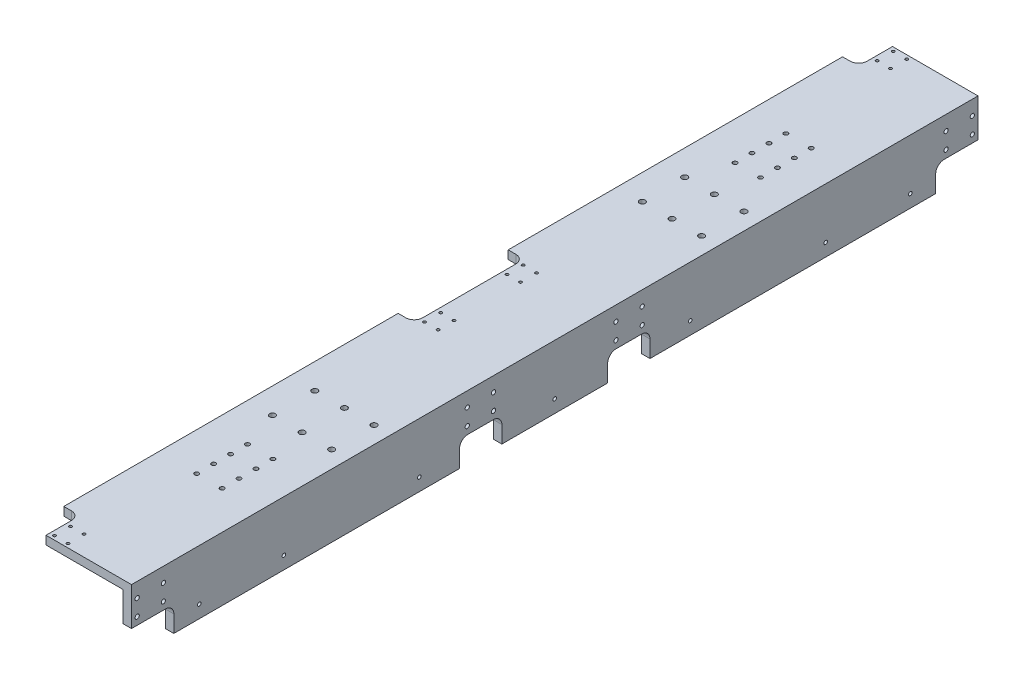
from build123d import *

# Parameters (mm, degrees)
EXTRUDE_1_DEPTH     = 500
HOLE_WIZARD_M8_1_D  = 6.8
MOVE_FACE_1_BY      = 20
MOVE_FACE_2_BY      = 15
CHAMFER_1_SIZE      = 10
SKETCH_16_W         = 19
SKETCH_16_H         = 40
SKETCH_16_H_2       = 130
CUT_EXTRUDE_1_DEPTH = 516.388203202
SKETCH_17_W         = 50
SKETCH_17_H         = 30
CUT_EXTRUDE_2_DEPTH = 520.639297975
HOLE_WIZARD_M6_1_D  = 5
HOLE_WIZARD_M4_1_D  = 3.3
HOLE_WIZARD_M5_3_D  = 4.2
HOLE_WIZARD_M6_2_D  = 5
FILLET_1_R          = 10


with BuildPart() as part:
    # 草图1 → 凸台-拉伸1 (new, symmetric)
    with BuildSketch(Plane.XY):
        Polygon((0, 0), (100, 0), (100, -90), (90, -90), (90, -10), (0, -10), align=None)
    extrude(amount=EXTRUDE_1_DEPTH, both=True)

    # M8 螺纹孔1 (through all)
    with Locations(Plane(origin=(0, 0, 0), x_dir=(1, 0, 0), z_dir=(0, 1, 0))):
        with Locations((10, -193.5), (10, -243.5), (80, -193.5), (80, -243.5), (45, -243.5), (45, -193.5), (45, 193.5), (45, 243.5), (80, 243.5), (80, 193.5), (10, 243.5), (10, 193.5)):
            Hole(HOLE_WIZARD_M8_1_D / 2)

    # Move Face 1: a face moved outward by 20.0
    extrude(part.faces().sort_by_distance((0, -5, 0))[0], amount=MOVE_FACE_1_BY, dir=(-1, 0, 0))

    # Move Face 2: a face moved inward by 15.0
    extrude(part.faces().sort_by_distance((95, -90, 0))[0], amount=MOVE_FACE_2_BY, dir=(0, 1, 0), mode=Mode.SUBTRACT)

    # 倒角1
    chamfer_1_edges = [part.edges().sort_by_distance(p)[0] for p in [
        (95, -75, 500),
        (-20, -5, 500),
        (95, -75, -500),
        (-20, -5, -500),
    ]]
    chamfer(chamfer_1_edges, length=CHAMFER_1_SIZE)

    # 草图16 → 切除-拉伸1 (cut, through all)
    with BuildSketch(Plane(origin=(0, 0, 0), x_dir=(1, 0, 0), z_dir=(0, 1, 0))):
        with Locations((-10.5, -480)):
            Rectangle(SKETCH_16_W, SKETCH_16_H)
        with Locations((-10.5, 480)):
            Rectangle(SKETCH_16_W, SKETCH_16_H)
        with Locations((-10.5, 0)):
            Rectangle(SKETCH_16_W, SKETCH_16_H_2)
    extrude(amount=-CUT_EXTRUDE_1_DEPTH, mode=Mode.SUBTRACT)

    # 草图17 → 切除-拉伸2 (cut, through all)
    with BuildSketch(Plane(origin=(100, 0, 0), x_dir=(0, 0, -1), z_dir=(1, 0, 0))):
        with Locations((-475, -60)):
            Rectangle(SKETCH_17_W, SKETCH_17_H)
        with Locations((-87.5, -60)):
            Rectangle(SKETCH_17_W, SKETCH_17_H)
        with Locations((87.5, -60)):
            Rectangle(SKETCH_17_W, SKETCH_17_H)
        with Locations((475, -60)):
            Rectangle(SKETCH_17_W, SKETCH_17_H)
    extrude(amount=-CUT_EXTRUDE_2_DEPTH, mode=Mode.SUBTRACT)

    # M6 螺纹孔1 (through all)
    with Locations(Plane(origin=(100, 0, 0), x_dir=(0, 0, -1), z_dir=(1, 0, 0))):
        with Locations((-493.3, -36.16903143), (-462.3, -36.16903143), (-493.3, -17.16903143), (-462.3, -17.16903143), (-103.3, -36.16903143), (-72.3, -36.16903143), (-103.3, -17.16903143), (-72.3, -17.16903143), (72.3, -17.16903143), (103.3, -17.16903143), (72.3, -36.16903143), (103.3, -36.16903143), (462.3, -17.16903143), (493.3, -17.16903143), (462.3, -36.16903143), (493.3, -36.16903143)):
            Hole(HOLE_WIZARD_M6_1_D / 2)

    # M4 螺纹孔1 (through all)
    with Locations(Plane(origin=(0, 0, 0), x_dir=(1, 0, 0), z_dir=(0, 1, 0))):
        with Locations((4.45210522, -476.4), (20.35210522, -476.4), (4.45210522, -495.4), (20.35210522, -495.4), (4.45210522, -39.2), (4.45210522, -58.2), (20.35210522, -58.2), (20.35210522, -39.2), (20.35210522, 39.2), (20.35210522, 58.2), (4.45210522, 58.2), (4.45210522, 39.2), (20.35210522, 495.4), (4.45210522, 495.4), (20.35210522, 476.4), (4.45210522, 476.4)):
            Hole(HOLE_WIZARD_M4_1_D / 2)

    # M5 螺纹孔3 (through all)
    with Locations(Plane(origin=(100, 0, 0), x_dir=(0, 0, -1), z_dir=(1, 0, 0))):
        with Locations((-420, -60), (-320, -60), (-160, -60), (0, -60), (160, -60), (320, -60), (420, -60)):
            Hole(HOLE_WIZARD_M5_3_D / 2)

    # M6 螺纹孔2 (through all)
    with Locations(Plane(origin=(0, 0, 0), x_dir=(1, 0, 0), z_dir=(0, 1, 0))):
        with Locations((25, -288), (55, -288), (25, -308), (55, -308), (25, -328), (55, -328), (25, -348), (55, -348), (55, 348), (25, 348), (55, 328), (25, 328), (55, 308), (25, 308), (55, 288), (25, 288)):
            Hole(HOLE_WIZARD_M6_2_D / 2)

    # 圆角1
    fillet_1_edges = [part.edges().sort_by_distance(p)[0] for p in [
        (-1, -5, 460),
        (-1, -5, -460),
        (-1, -5, -65),
        (-1, -5, 65),
        (95, -45, 450),
        (95, -45, -62.5),
        (95, -45, -112.5),
        (95, -45, -450),
        (95, -45, 112.5),
        (95, -45, 62.5),
    ]]
    fillet(fillet_1_edges, radius=FILLET_1_R)


solid = part.part
